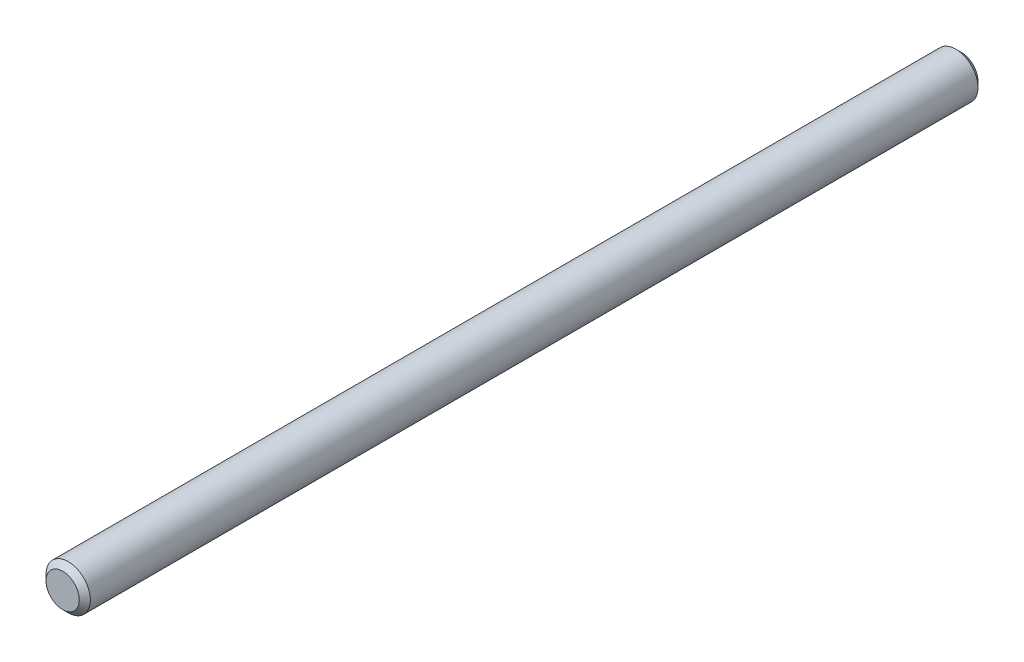
from build123d import *

# Parameters (mm, degrees)
SKETCH1_R           = 0.4
BOSS_EXTRUDE1_DEPTH = 16.2
CHAMFER1_SIZE       = 0.1


with BuildPart() as part:
    # Sketch1 → Boss-Extrude1 (new body)
    with BuildSketch(Plane.XY):
        Circle(SKETCH1_R)
    extrude(amount=BOSS_EXTRUDE1_DEPTH)

    # Chamfer1
    chamfer1_edges = [part.edges().sort_by_distance(p)[0] for p in [
        (-0.4, 0, 0),
        (-0.4, 0, 16.2),
    ]]
    chamfer(chamfer1_edges, length=CHAMFER1_SIZE)


solid = part.part
